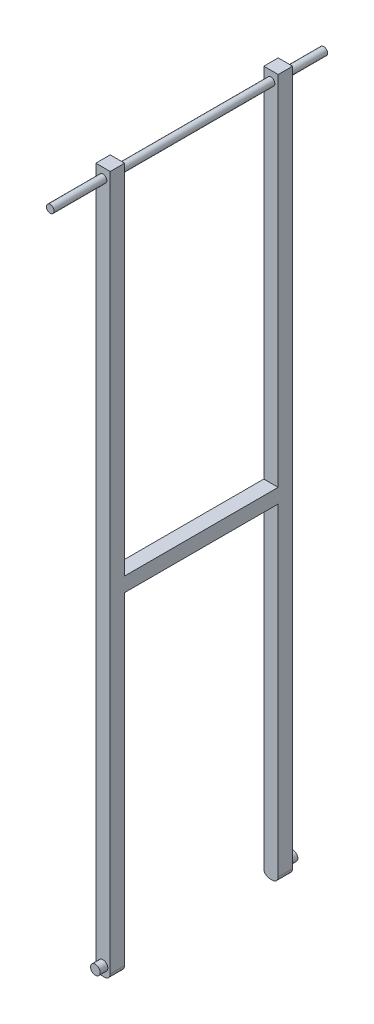
from build123d import *

# Parameters (mm, degrees)
SKETCH1_W                = 15
SKETCH1_H                = 15
BOSS_EXTRUDE1_DEPTH      = 730
SKETCH2_R                = 5
BOSS_EXTRUDE2_DEPTH      = 8
SKETCH4_W                = 15
SKETCH4_H                = 15
BOSS_EXTRUDE3_DEPTH      = 160
SKETCH5_W                = 15
SKETCH5_H                = 730
BOSS_EXTRUDE4_DEPTH      = 15
BOSS_EXTRUDE5_START      = 8
SKETCH6_R                = 5
BOSS_EXTRUDE5_DEPTH      = 8
FILLET1_R                = 6
BOSS_EXTRUDE6_DEPTH      = 230
BOSS_EXTRUDE6_DEPTH_BACK = 55
SKETCH7_R                = 4


with BuildPart() as part:
    # Sketch1 → Boss-Extrude1 (new body)
    with BuildSketch(Plane(origin=(0, 0, 0), x_dir=(1, 0, 0), z_dir=(0, 1, 0))):
        Rectangle(SKETCH1_W, SKETCH1_H)
    extrude(amount=BOSS_EXTRUDE1_DEPTH)

    # Sketch2 → Boss-Extrude2 (add)
    with BuildSketch(Plane(origin=(0, 0, -7.5), x_dir=(-1, 0, 0), z_dir=(0, 0, -1))):
        with Locations(Location((0, 10, 0), (0, 0, 180))):
            Circle(SKETCH2_R)
    extrude(amount=BOSS_EXTRUDE2_DEPTH)

    # Sketch4 → Boss-Extrude3 (add)
    with BuildSketch(Plane.XY.offset(7.5)):
        with Locations((0, 350)):
            Rectangle(SKETCH4_W, SKETCH4_H)
    extrude(amount=BOSS_EXTRUDE3_DEPTH)

    # Sketch5 → Boss-Extrude4 (add)
    with BuildSketch(Plane.XY.offset(167.5)):
        with Locations((0, 365)):
            Rectangle(SKETCH5_W, SKETCH5_H)
    extrude(amount=BOSS_EXTRUDE4_DEPTH)

    # Sketch6 → Boss-Extrude5 (add)
    with BuildSketch(Plane.XY.offset(182.5).offset(BOSS_EXTRUDE5_START)):
        with Locations((0, 10)):
            Circle(SKETCH6_R)
    extrude(amount=-BOSS_EXTRUDE5_DEPTH)

    # Fillet1
    fillet1_edges = [part.edges().sort_by_distance(p)[0] for p in [
        (7.5, 0, 175),
        (-7.5, 0, 175),
        (-7.5, 0, 0),
        (7.5, 0, 0),
    ]]
    fillet(fillet1_edges, radius=FILLET1_R)

    # Sketch7 → Boss-Extrude6 (add, two sides: drawn at the far end of the back side and taken through both)
    with BuildSketch(Plane.XY.offset(7.5).offset(-BOSS_EXTRUDE6_DEPTH_BACK)):
        with Locations((0, 720)):
            Circle(SKETCH7_R)
    extrude(amount=BOSS_EXTRUDE6_DEPTH + BOSS_EXTRUDE6_DEPTH_BACK)


solid = part.part
